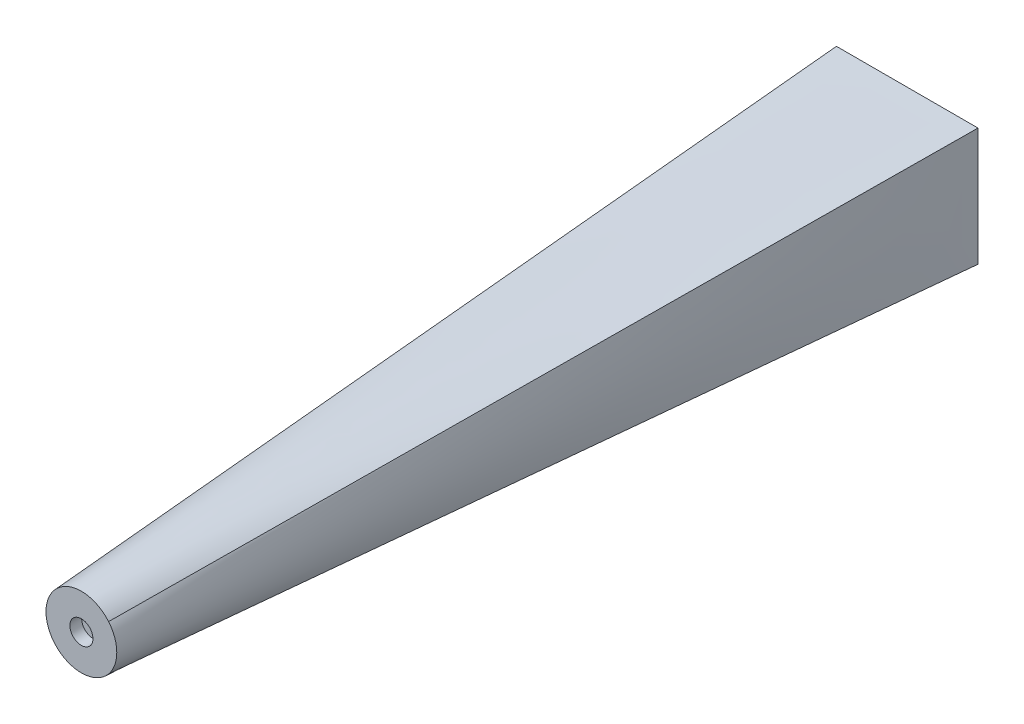
SolidWorks part; units mm, degrees
ref_plane "前视基准面" through (0, 0, 0) normal (0, 0, 1) x (1, 0, 0)
ref_plane "上视基准面" through (0, 0, 0) normal (0, 1, 0) x (1, 0, 0)
ref_plane "右视基准面" through (0, 0, 0) normal (1, 0, 0) x (0, 0, -1)
sketch "草图1" plane through (0, 0, 0) normal (0, 0, 1) x (1, 0, 0)
  circle A0 centre (0, 0) radius 15
  dimension "D1" = 30
ref_plane "基准面1" through (0, 0, -350) normal (0, 0, 1) x (1, 0, 0)
sketch "草图2" plane through (0, 0, -350) normal (0, 0, 1) x (1, 0, 0)
  line L1 (-30, 25) -> (30, 25)
  line L2 (-30, 25) -> (-30, -25)
  line L3 (-30, -25) -> (30, -25)
  line L4 (30, 25) -> (30, -25)
  line L5 (-30, 25) -> (30, -25) construction
  line L6 (-30, -25) -> (30, 25) construction
  dimension "D2" = 60
  dimension "D3" = 50
loft "放样1" add profiles "草图2", "草图1"
sketch "草图3" plane through (0, 0, 0) normal (0, 0, 1) x (1, 0, 0)
  circle A0 centre (0, 0) radius 4.8895
extrude "切除-拉伸1" cut sketch "草图3" against normal blind 5
